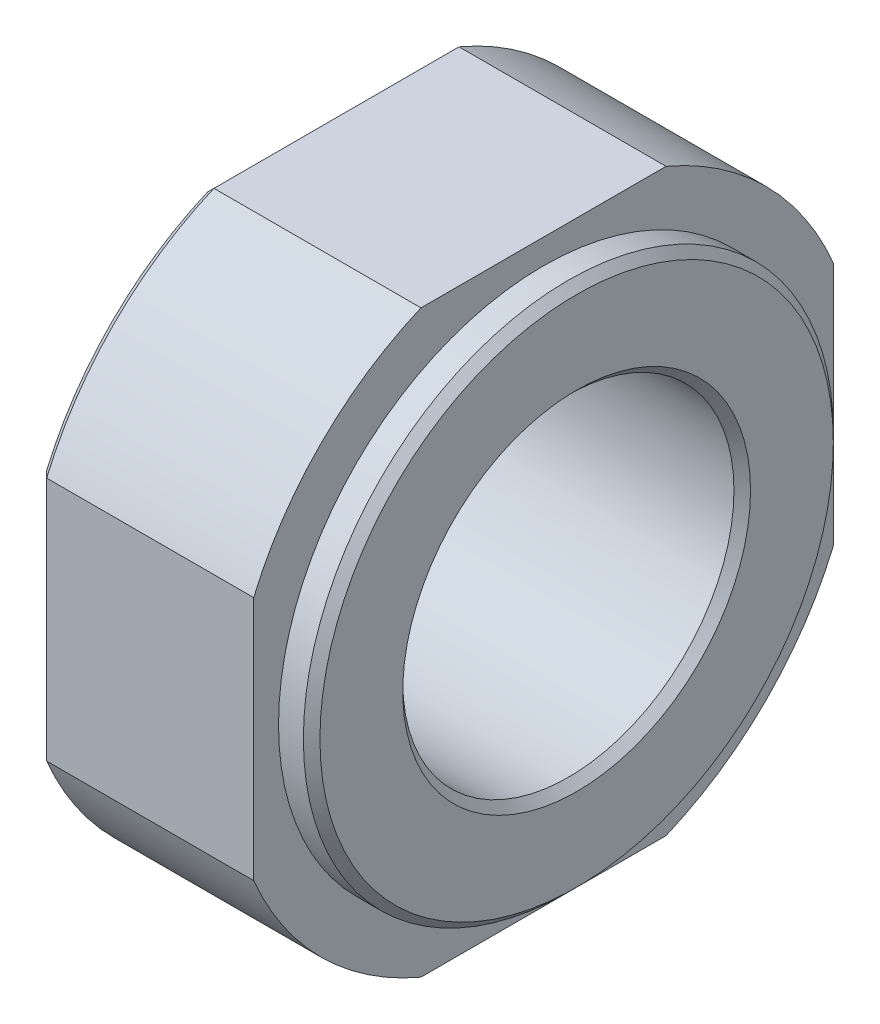
SolidWorks part; units mm, degrees
material "S45C"
ref_plane "Front Plane" through (0, 0, 0) normal (0, 0, 1) x (1, 0, 0)
ref_plane "Top Plane" through (0, 0, 0) normal (0, 1, 0) x (1, 0, 0)
ref_plane "Right Plane" through (0, 0, 0) normal (1, 0, 0) x (0, 0, -1)
sketch "Sketch1" plane through (0, 0, 0) normal (1, 0, 0) x (0, 0, -1)
  circle A0 centre (0, 0) radius 10
  circle A1 centre (0, 0) radius 19
  dimension "D1" = 38
  dimension "D2" = 20
extrude "Boss-Extrude1" add sketch "Sketch1" along normal blind 15
cosmetic thread "Cosmetic Thread1" parameters "D2"=24
sketch "Sketch2" plane through (15, 0, 0) normal (1, 0, 0) x (0, 0, -1)
  circle A0 centre (0, 0) radius 16
  dimension "D1" = 32
extrude "Cut-Extrude1" cut sketch "Sketch2" against normal blind 2 flip side to cut
sketch "Sketch3" plane through (0, 0, 0) normal (-1, 0, 0) x (0, 0, 1)
  line L1 (-17.5, -17.5) -> (17.5, -17.5)
  line L2 (-17.5, -17.5) -> (-17.5, 17.5)
  line L3 (-17.5, 17.5) -> (17.5, 17.5)
  line L4 (17.5, -17.5) -> (17.5, 17.5)
  line L5 (-17.5, -17.5) -> (17.5, 17.5) construction
  line L6 (-17.5, 17.5) -> (17.5, -17.5) construction
  point P0 (0, 0)
  dimension "D1" = 35
  dimension "D2" = 35
extrude "Cut-Extrude2" cut sketch "Sketch3" against normal through all flip side to cut
chamfer "Chamfer1" distance 0.5 angle 45 11 edges at (0, -13.435, 13.435) (0, -17.5, 0) (0, -13.435, -13.435) (0, 0, -17.5) (0, 13.435, -13.435) (0, 17.5, 0) (0, 13.435, 13.435) (0, 0, 17.5) (0, 0, -10) (15, 0, -16) (15, 0, -10)
